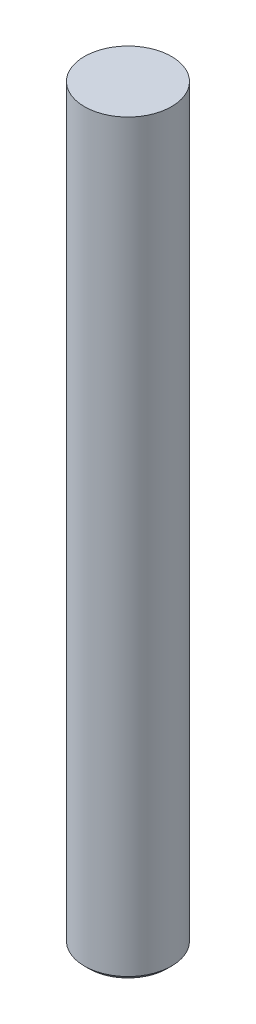
from build123d import *

# Parameters (mm, degrees)
SKETCH2_R           = 10
BOSS_EXTRUDE1_DEPTH = 172
CHAMFER1_SIZE       = 1


with BuildPart() as part:
    # Sketch2 → Boss-Extrude1 (new body)
    with BuildSketch(Plane(origin=(0, 0, 0), x_dir=(1, 0, 0), z_dir=(0, 1, 0))):
        with Locations(Location((0, 0, 0), (0, 0, 270))):
            Circle(SKETCH2_R)
    extrude(amount=BOSS_EXTRUDE1_DEPTH)

    # Chamfer1
    chamfer1_edges = [part.edges().sort_by_distance(p)[0] for p in [
        (0, 0, -10),
    ]]
    chamfer(chamfer1_edges, length=CHAMFER1_SIZE)


solid = part.part
